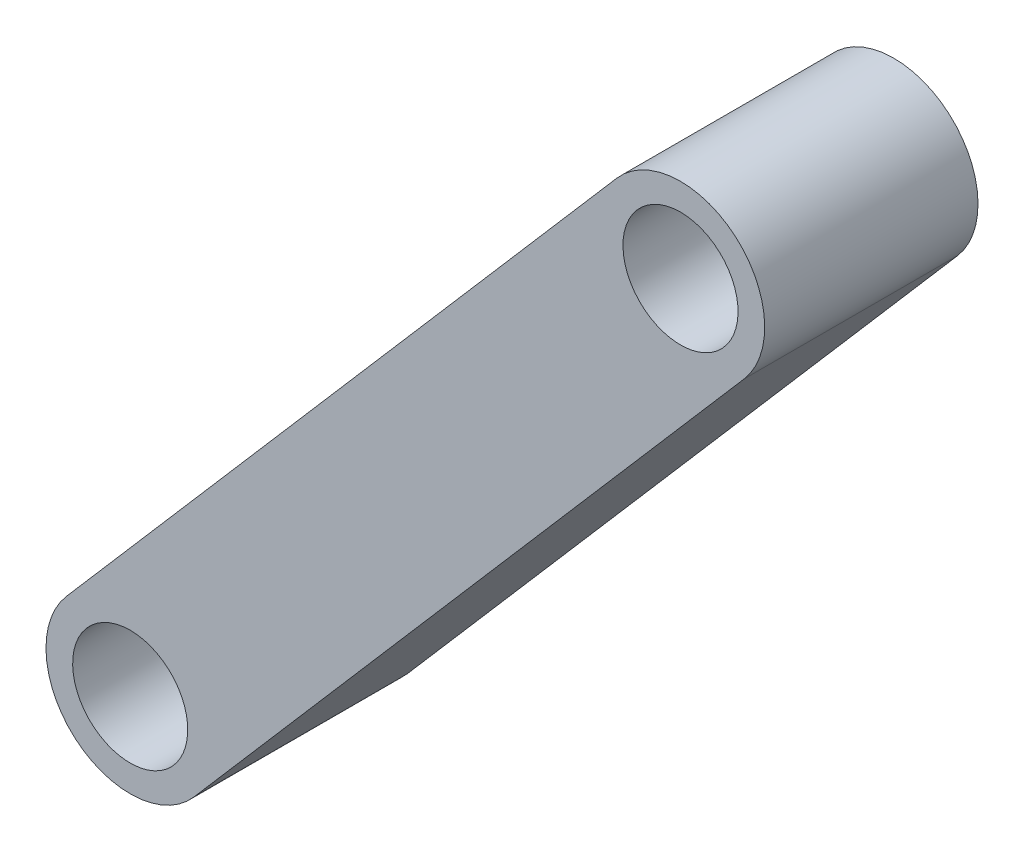
from build123d import *

# Parameters (mm, degrees)
SKETCH1_R           = 2.6035
BOSS_EXTRUDE1_DEPTH = 9.652


with BuildPart() as part:
    # Sketch1 → Boss-Extrude1 (new body)
    with BuildSketch(Plane.XY):
        with BuildLine():
            Line((12.356395011, -0.759834892), (37.258046093, 28.076215001))
            ThreePointArc((37.258046093, 28.076215001), (42.63181619, 28.469654882), (43.025256071, 23.095884784))
            Line((43.025256071, 23.095884784), (18.123604989, -5.740165108))
            ThreePointArc((18.123604989, -5.740165108), (12.749834892, -6.133604989), (12.356395011, -0.759834892))
        make_face()
        with Locations(Location((15.24, -3.25, 0), (0, 0, 90))):
            Circle(SKETCH1_R, mode=Mode.SUBTRACT)
        with Locations(Location((40.141651082, 25.586049892, 0), (0, 0, 90))):
            Circle(SKETCH1_R, mode=Mode.SUBTRACT)
    extrude(amount=BOSS_EXTRUDE1_DEPTH)


solid = part.part
